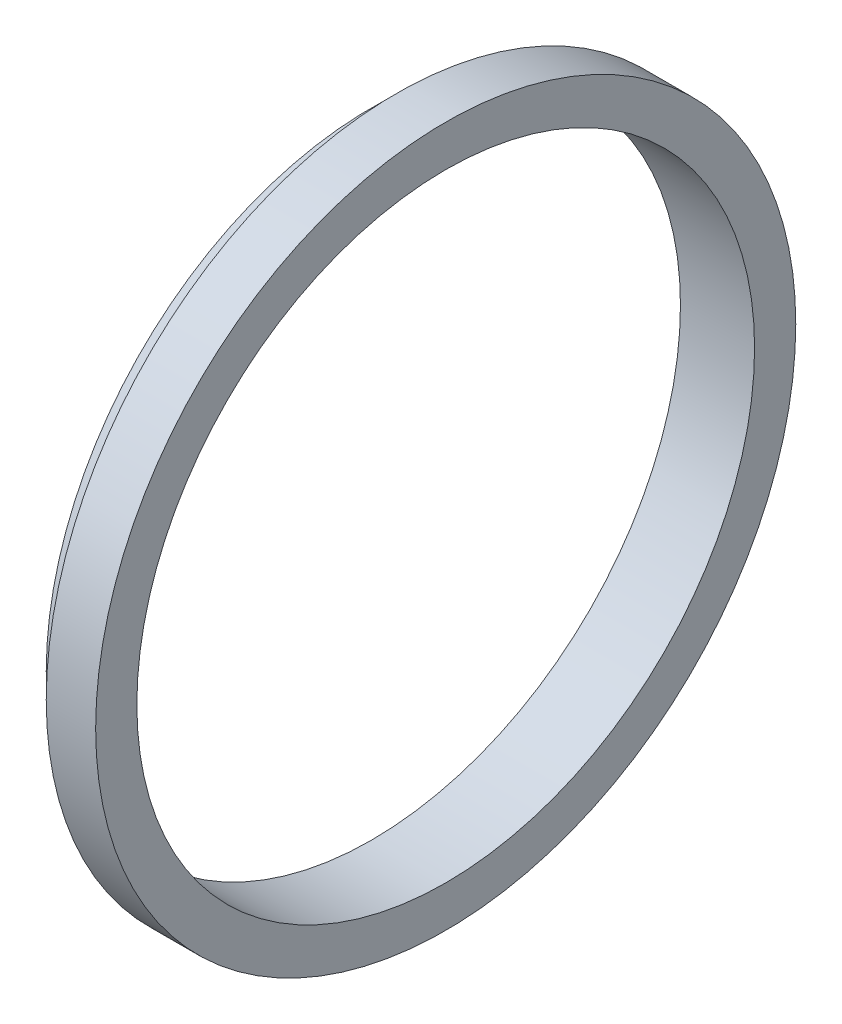
from build123d import *


with BuildPart() as part:
    # 草图1 → 旋转1 (revolve)
    with BuildSketch(Plane.XY, mode=Mode.PRIVATE) as revolve_1_sk:
        Polygon((0, 37.5), (9, 37.5), (9, 42.5), (3, 42.5), (3, 40.5), (0, 39.5), align=None)
    revolve(revolve_1_sk.sketch.rotate(Axis((-9.114263851, 0, 0), (1, 0, 0)), 90), axis=Axis((-9.114263851, 0, 0), (1, 0, 0)))


solid = part.part
